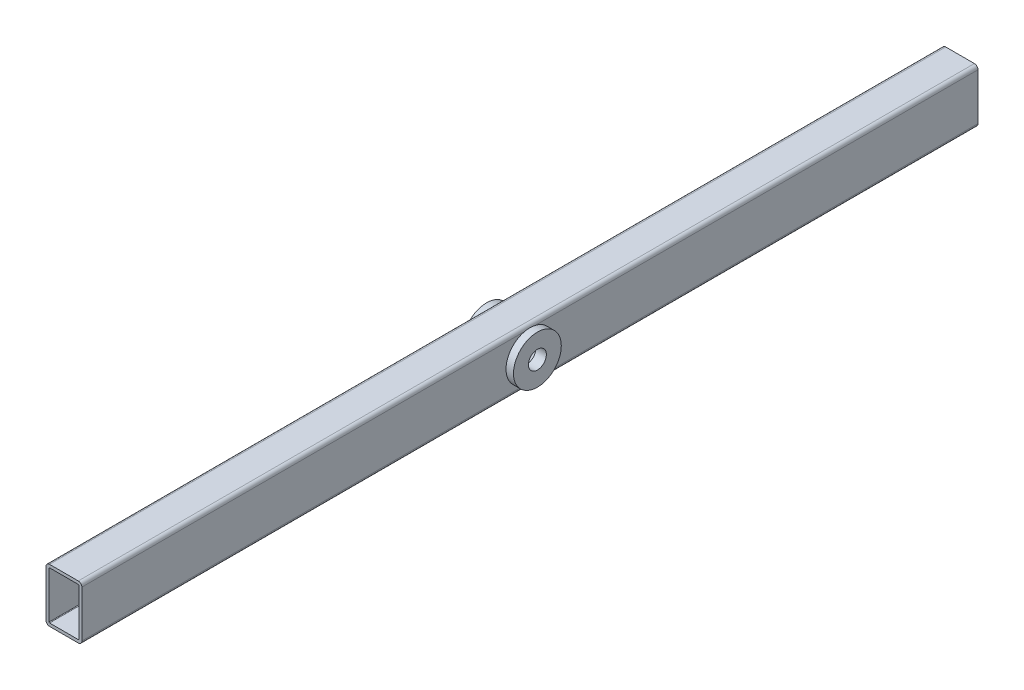
from build123d import *

# Parameters (mm, degrees)
BOSS_EXTRUDE_1_DEPTH     = 1500
CUT_EXTRUDE_1_DEPTH      = 1504.894943139
CUT_EXTRUDE_1_DEPTH_BACK = 1504.894943139
SKETCH_2_R               = 30
SKETCH_3_R               = 80
SKETCH_3_R_2             = 30
BOSS_EXTRUDE_2_DEPTH     = 25


with BuildPart() as part:
    # Sketch 1 → Boss-Extrude 1 (new, symmetric)
    with BuildSketch(Plane.XY):
        with BuildLine():
            Line((0, 90), (-48, 90))
            ThreePointArc((-48, 90), (-56.485281374, 86.485281374), (-60, 78))
            Line((-60, 78), (-60, 0))
            Line((-60, 0), (-60, -78))
            ThreePointArc((-60, -78), (-56.485281374, -86.485281374), (-48, -90))
            Line((-48, -90), (0, -90))
            Line((0, -90), (48, -90))
            ThreePointArc((48, -90), (56.485281374, -86.485281374), (60, -78))
            Line((60, -78), (60, 78))
            ThreePointArc((60, 78), (56.485281374, 86.485281374), (48, 90))
            Line((48, 90), (0, 90))
        make_face()
        with BuildLine():
            Line((0, 80), (-48, 80))
            ThreePointArc((-48, 80), (-49.414213562, 79.414213562), (-50, 78))
            Line((-50, 78), (-50, 0))
            Line((-50, 0), (-50, -78))
            ThreePointArc((-50, -78), (-49.414213562, -79.414213562), (-48, -80))
            Line((-48, -80), (0, -80))
            Line((0, -80), (48, -80))
            ThreePointArc((48, -80), (49.414213562, -79.414213562), (50, -78))
            Line((50, -78), (50, 78))
            ThreePointArc((50, 78), (49.414213562, 79.414213562), (48, 80))
            Line((48, 80), (0, 80))
        make_face(mode=Mode.SUBTRACT)
    extrude(amount=BOSS_EXTRUDE_1_DEPTH, both=True)

    # Sketch 2 → Cut-Extrude 1 (cut, two sides: drawn at the far end of the back side and taken through both)
    with BuildSketch(Plane(origin=(0, 0, 0), x_dir=(0, 0, -1), z_dir=(1, 0, 0)).offset(-CUT_EXTRUDE_1_DEPTH_BACK)):
        Circle(SKETCH_2_R)
    extrude(amount=CUT_EXTRUDE_1_DEPTH + CUT_EXTRUDE_1_DEPTH_BACK, mode=Mode.SUBTRACT)

    # Sketch 3 → Boss-Extrude 2 (add)
    with BuildSketch(Plane(origin=(60, 0, 0), x_dir=(0, 0, -1), z_dir=(1, 0, 0))):
        with Locations(Location((0, 0, 0), (0, 0, 102.838568141))):
            Circle(SKETCH_3_R)
        Circle(SKETCH_3_R_2, mode=Mode.SUBTRACT)
    boss_extrude_2 = extrude(amount=BOSS_EXTRUDE_2_DEPTH)

    # Mirror 1: Boss-Extrude 2 across plane
    add(boss_extrude_2.mirror(Plane(origin=(0, 0, 0), x_dir=(0, 0, 1), z_dir=(1, 0, 0))))


solid = part.part
